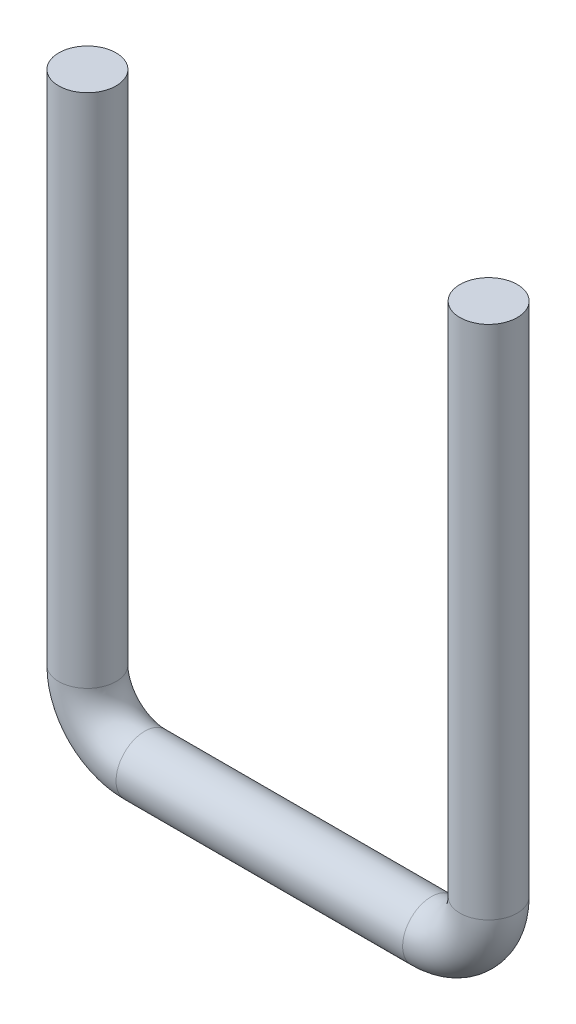
SolidWorks part; units mm, degrees
material "Q235B"
ref_plane "Front Plane" through (0, 0, 0) normal (0, 0, 1) x (1, 0, 0)
ref_plane "Top Plane" through (0, 0, 0) normal (0, 1, 0) x (1, 0, 0)
ref_plane "Right Plane" through (0, 0, 0) normal (1, 0, 0) x (0, 0, -1)
sketch "Sketch1" plane through (0, 0, 0) normal (0, 0, 1) x (1, 0, 0)
  line L0 (-35, 100) -> (-35, 10)
  line L1 (-25, 0) -> (25, 0)
  line L2 (0, 0) -> (0, 192.3395) construction
  line L3 (35, 100) -> (35, 10)
  arc A0 (35, 10) -> (25, 0) centre (25, 10) cw
  arc A1 (-35, 10) -> (-25, 0) centre (-25, 10) ccw
  point P9 (35, 0)
  point P12 (-35, 0)
  dimension "D3" = 10
  dimension "D1" = 70
  dimension "D2" = 100
sweep "Sweep1" add path "Sketch1" circular profile diameter 10 parameters "D3"=10
cosmetic thread "Cosmetic Thread1"
cosmetic thread "Cosmetic Thread2"
